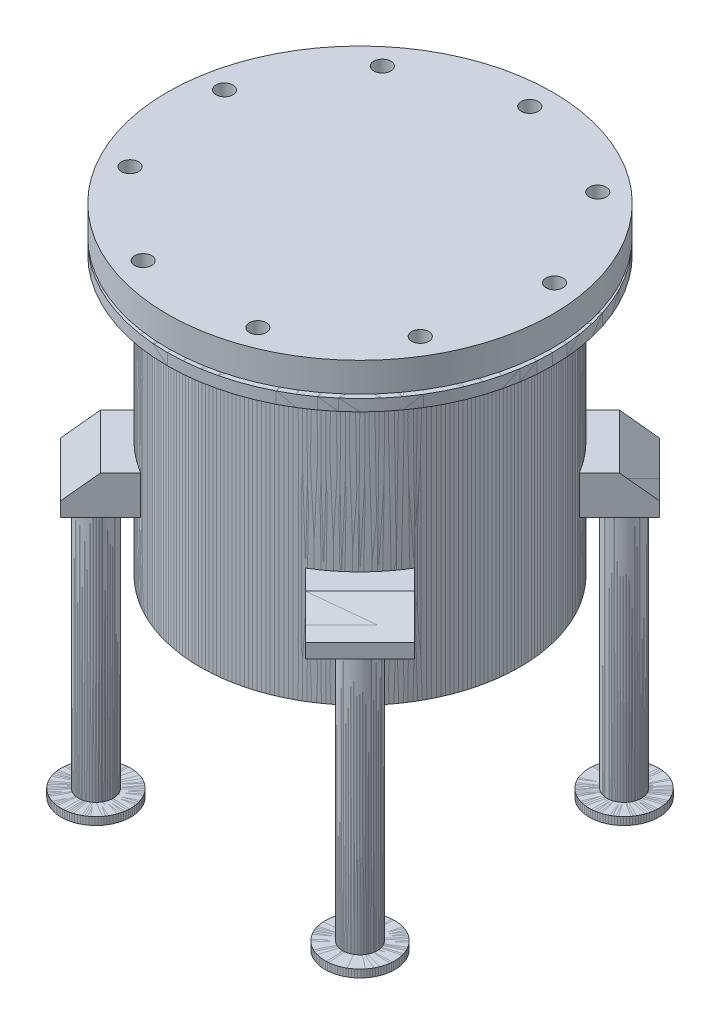
SolidWorks part; units mm, degrees
material "AISI 304"
ref_plane "Front Plane" through (0, 0, 0) normal (0, 0, 1) x (1, 0, 0)
ref_plane "Top Plane" through (0, 0, 0) normal (0, 1, 0) x (1, 0, 0)
ref_plane "Right Plane" through (0, 0, 0) normal (1, 0, 0) x (0, 0, -1)
sketch "Sketch1" plane through (0, 0, 0) normal (0, 1, 0) x (1, 0, 0)
  circle A0 centre (0, 0) radius 415
  dimension "D1" = 830
extrude "Boss-Extrude1" add sketch "Sketch1" along normal blind 750
shell "Shell1" thickness 15
sketch "Sketch2" plane through (0, 750, 0) normal (0, 1, 0) x (1, 0, 0)
  circle A0 centre (0, 0) radius 415 construction
  circle A1 centre (0, 0) radius 415
  circle A2 centre (0, 0) radius 500
  dimension "D1" = 1000
extrude "Boss-Extrude2" add sketch "Sketch2" against normal blind 30
sketch "Sketch3" plane through (0, 750, 0) normal (0, 1, 0) x (1, 0, 0)
  circle A0 centre (0, 0) radius 500
extrude "Boss-Extrude3" add sketch "Sketch3" along normal blind 86 separate body
sketch "Sketch4" plane through (0, 0, 0) normal (0, 0, 1) x (1, 0, 0)
  line L1 (-500, 750) -> (553.2519, 750)
  line L2 (-500, 750) -> (-500, 760)
  line L3 (-500, 760) -> (553.2519, 760)
  line L4 (553.2519, 750) -> (553.2519, 760)
  dimension "D1" = 10
extrude "Cut-Extrude1" cut sketch "Sketch4" against normal through all both and the other way through all
ref_plane "Plane1" through (0, 300, 0) normal (0, -1, 0) x (-1, 0, 0)
sketch "Sketch5" plane through (0, 300, 0) normal (0, -1, 0) x (-1, 0, 0)
  line L0 (355.5132, -214.0919) -> (459.6194, -318.1981)
  line L1 (-459.6194, 318.1981) -> (-355.5132, 214.0919)
  line L2 (-459.6194, 318.1981) -> (-318.1981, 459.6194)
  line L3 (-318.1981, 459.6194) -> (-214.0919, 355.5132)
  line L4 (318.1981, -459.6194) -> (459.6194, -318.1981)
  line L5 (0, 0) -> (0, 308.9365) construction
  line L6 (0, 0) -> (-404.8921, 404.8921) construction
  line L7 (214.0919, -355.5132) -> (318.1981, -459.6194)
  circle A0 centre (0, 0) radius 415 construction
  arc A1 (-214.0919, 355.5132) -> (-355.5132, 214.0919) centre (0, 0) ccw
  arc A2 (214.0919, -355.5132) -> (355.5132, -214.0919) centre (0, 0) ccw
  dimension "D1" = 200
  dimension "D2" = 1100
  dimension "D3" = 45
extrude "Boss-Extrude4" add sketch "Sketch5" along normal blind 100
sketch "Sketch6" plane through (70.7107, 0, 70.7107) normal (0.7071, 0, 0.7071) x (0.7071, 0, -0.7071)
  line L0 (-550, 300) -> (-550, 237.0832)
  line L1 (-550, 200) -> (-550, 300) construction
  line L2 (-550, 237.0832) -> (-476.3858, 300)
  line L3 (-402.7716, 300) -> (-550, 300) construction
  line L4 (-476.3858, 300) -> (-550, 300)
  line L5 (0, 0) -> (0, 349.0255) construction
  line L6 (-415, 0) -> (415, 0) construction
  line L7 (550, 237.0832) -> (476.3858, 300)
  line L8 (550, 300) -> (550, 237.0832)
  line L9 (476.3858, 300) -> (550, 300)
extrude "Cut-Extrude2" cut sketch "Sketch6" against normal through all both and the other way through all
sketch "Sketch7" plane through (0, 200, 0) normal (0, -1, 0) x (1, 0, 0)
  line L0 (0, 0) -> (-388.9087, 388.9087) construction
  line L2 (0, 0) -> (0, 668.833) construction
  line L3 (-318.1981, 459.6194) -> (-459.6194, 318.1981) construction
  line L4 (0, 0) -> (431.5008, 431.5008) construction
  circle A0 centre (-342.9468, 342.9468) radius 45
  circle A1 centre (342.9468, -342.9468) radius 45
  dimension "D1" = 90
  dimension "D2" = 65
extrude "Boss-Extrude5" add sketch "Sketch7" along normal blind 700
sketch "Sketch8" plane through (0, -500, 0) normal (0, -1, 0) x (1, 0, 0)
  circle A0 centre (-342.9468, 342.9468) radius 90.376
  circle A1 centre (342.9468, -342.9468) radius 90.376
extrude "Boss-Extrude6" add sketch "Sketch8" against normal blind 20
sketch "Sketch9" plane through (0, 836, 0) normal (0, 1, 0) x (1, 0, 0)
  circle A0 centre (2.8028, 438.0623) radius 22.1853
extrude "Cut-Extrude3" cut sketch "Sketch9" against normal blind 136
pattern_circular "CirPattern1" count 9 over 360 about axis through (0, 0, 0) along (0, 1, 0) of "Cut-Extrude3"
pattern_circular "CirPattern5" count 4 over 360 about axis through (0, 0, 0) along (0, 1, 0) of bodies 131
sketch "Sketch10" plane through (0, 0, 0) normal (1, 0, 0) x (0, 0, -1)
  line L0 (-433.3228, -500) -> (-252.5708, -500) construction
  circle A0 centre (0, 500) radius 15
  dimension "D1" = 30
  dimension "D2" = 1000
extrude "Cut-Extrude4" cut sketch "Sketch10" against normal blind 722
